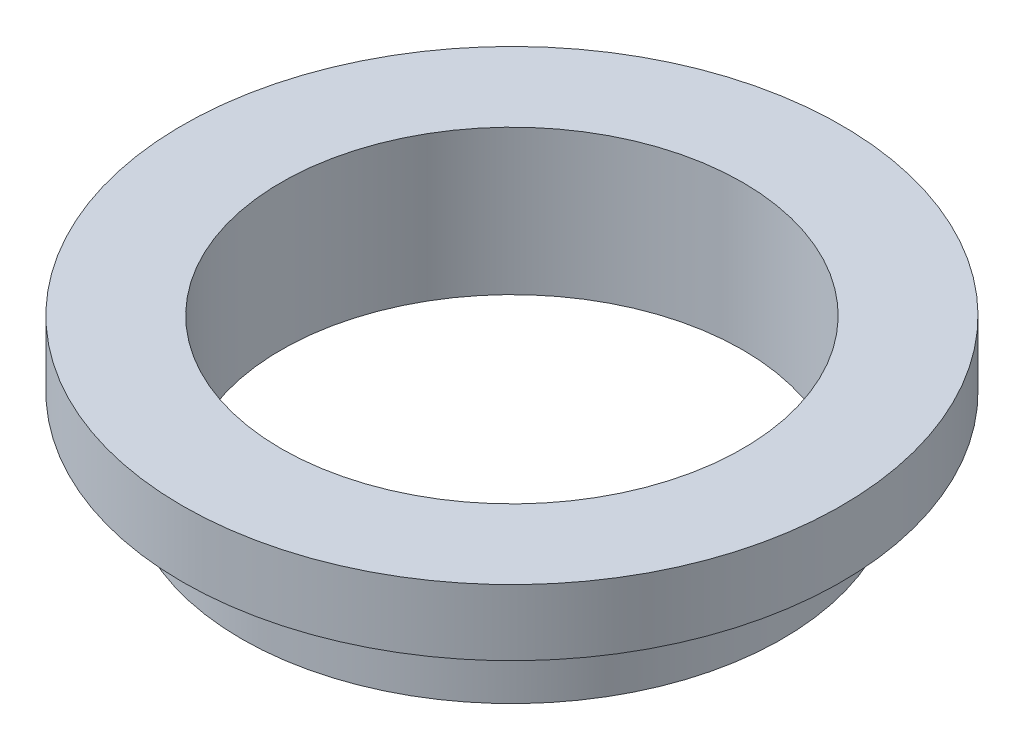
SolidWorks part; units mm, degrees
ref_plane "前视基准面" through (0, 0, 0) normal (0, 0, 1) x (1, 0, 0)
ref_plane "上视基准面" through (0, 0, 0) normal (0, 1, 0) x (1, 0, 0)
ref_plane "右视基准面" through (0, 0, 0) normal (1, 0, 0) x (0, 0, -1)
sketch "草图1" plane through (0, 0, 0) normal (1, 0, 0) x (0, 0, -1)
  line L0 (0, 46.2717) -> (0, -46.2717) construction
  line L2 (17.5, 0) -> (17.5, 11)
  line L3 (17.5, 11) -> (25, 11)
  line L4 (25, 11) -> (25, 6)
  line L5 (25, 6) -> (20.5, 6)
  line L6 (20.5, 6) -> (20.5, 0)
  line L7 (20.5, 0) -> (17.5, 0)
revolve "旋转1" add sketch "草图1" angle 360 about L0
